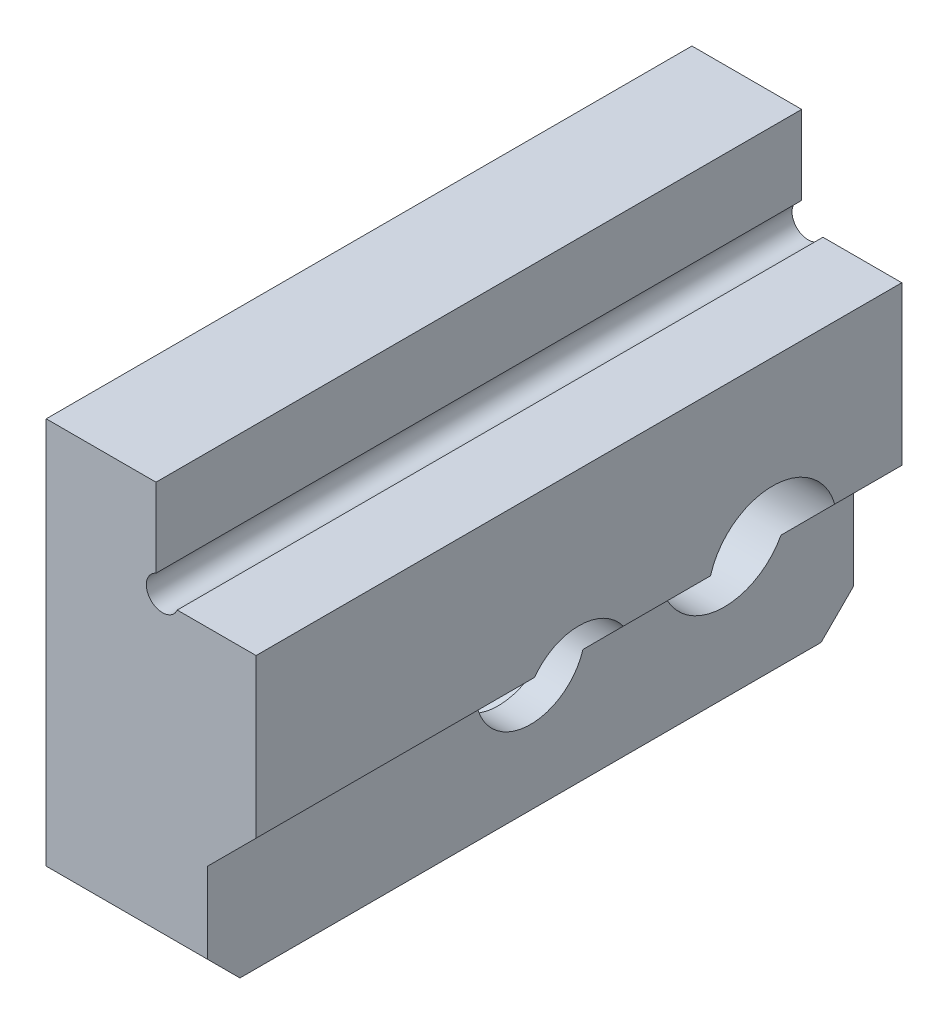
SolidWorks part; units mm, degrees
ref_plane "Front Plane" through (0, 0, 0) normal (0, 0, 1) x (1, 0, 0)
ref_plane "Top Plane" through (0, 0, 0) normal (0, 1, 0) x (1, 0, 0)
ref_plane "Right Plane" through (0, 0, 0) normal (1, 0, 0) x (0, 0, -1)
sketch "Sketch1" plane through (0, 0, 0) normal (0, 0, 1) x (1, 0, 0)
  line L0 (0, 0) -> (0, 13)
  line L1 (0, 13) -> (3.4, 13)
  line L2 (3.4, 13) -> (3.4, 10.5583)
  line L3 (4.0583, 9.9) -> (6.5, 9.9)
  line L4 (6.5, 9.9) -> (6.5, 0)
  line L5 (6.5, 0) -> (0, 0)
  arc A0 (3.4, 10.5583) -> (4.0583, 9.9) centre (3.6, 10.1) ccw
  dimension "D7" = 1
  dimension "D1" = 3.1
  dimension "D2" = 3.1
  dimension "D3" = 13
  dimension "D4" = 6.5
  dimension "D5" = 0.2
  dimension "D6" = 0.2
extrude "Boss-Extrude1" add sketch "Sketch1" along normal blind 20
sketch "Sketch7" plane through (0, 0, 20) normal (0, 0, 1) x (1, 0, 0)
  line L0 (6.5, 5) -> (5, 3.5)
  line L1 (6.5, 0) -> (6.5, 9.9) construction
  line L2 (5, 3.5) -> (5, 0)
  line L3 (0, 0) -> (6.5, 0) construction
  line L4 (5, 0) -> (6.5, 0)
  line L5 (6.5, 0) -> (6.5, 5)
  dimension "D1" = 1.5
  dimension "D2" = 45
  dimension "D3" = 3.5
extrude "Cut-Extrude1" cut sketch "Sketch7" against normal up to surface (20 mm away) up to face at (3.3394, 7.9822, 0)
hole_wizard "Hole size per socket head cap screw type 0" positions "Sketch5" profile "Sketch6" counterbore size "M3" standard "GB"
sketch "Sketch5" plane through (0, 0, 0) normal (1, 0, 0) x (0, 0, -1)
  line L0 (-20, 0) -> (0, 0) construction
  line L1 (-10, 0) -> (-10, 2.1068) construction
  line L2 (-20, 0) -> (0, 0) construction
  point P0 (-10, 4)
  dimension "D2" = 4
sketch "Sketch6" plane through (0, 4, 10) normal (0, 1, 0) x (0, 0, 1)
  line L0 (0, 0) -> (0, 11.0215)
  line L1 (0, 11.0215) -> (1.7, 10)
  line L2 (1.7, 10) -> (1.7, 4)
  line L3 (1.7, 4) -> (3, 4)
  line L4 (3, 4) -> (3, 0)
  line L5 (3, 0) -> (0, 0)
  line L10 (0, 11.0215) -> (-1.7, 10) construction
  line L11 (0, -6.35) -> (0, 107.95) construction
  dimension "孔直径" = 3.4
  dimension "孔深度" = 10
  dimension "柱形沉头孔直径" = 6
  dimension "柱形沉头孔深度" = 4
  dimension "导头角度" = 118
chamfer "Chamfer1" distance 1 angle 45 2 edges at (2.5, 0, 20) (2.5, 0, 0)
sketch "Sketch8" plane through (0, 0, 0) normal (-1, 0, 0) x (0, 0, 1)
  circle A0 centre (4, 4.45) radius 2
  dimension "D1" = 4
extrude "Cut-Extrude2" cut sketch "Sketch8" against normal blind 8
